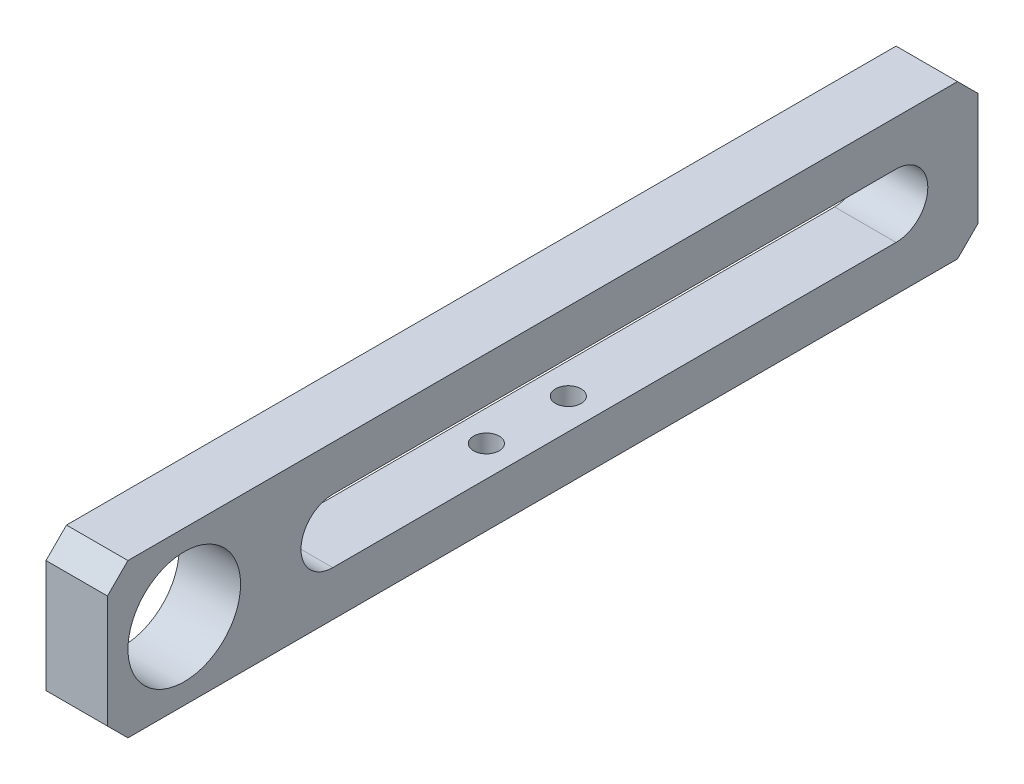
from build123d import *

# Parameters (mm, degrees)
SKETCH1_W              = 85
SKETCH1_H              = 15
EXTRUDE1_DEPTH         = 6
M12X1_0_TAPPED_HOLE1_D = 11
CHAMFER1_SIZE          = 2
M3_TAPPED_HOLE1_D      = 2.5
M3_TAPPED_HOLE1_DEPTH  = 8.5
M3_TAPPED_HOLE1_TIP    = 0.751075774


with BuildPart() as part:
    # Sketch1 → Extrude1 (new body)
    with BuildSketch(Plane(origin=(0, 0, 0), x_dir=(0, 0, -1), z_dir=(1, 0, 0))):
        with Locations((42.5, -7.5)):
            Rectangle(SKETCH1_W, SKETCH1_H)
        with BuildLine():
            Line((22, -4.4), (77, -4.4))
            ThreePointArc((77, -4.4), (80.1, -7.5), (77, -10.6))
            Line((77, -10.6), (22, -10.6))
            ThreePointArc((22, -10.6), (18.9, -7.5), (22, -4.4))
        make_face(mode=Mode.SUBTRACT)
    extrude(amount=EXTRUDE1_DEPTH)

    # M12x1.0 Tapped Hole1 (through all)
    with Locations(Plane(origin=(6, 0, 0), x_dir=(0, 0, -1), z_dir=(1, 0, 0))):
        with Locations((7.5, -7.5)):
            Hole(M12X1_0_TAPPED_HOLE1_D / 2)

    # Chamfer1
    chamfer1_edges = [part.edges().sort_by_distance(p)[0] for p in [
        (3, 0, 0),
        (3, 0, -85),
        (3, -15, -85),
        (3, -15, 0),
    ]]
    chamfer(chamfer1_edges, length=CHAMFER1_SIZE)

    # M3 Tapped Hole1
    with Locations(Plane.XZ.offset(15)):
        with Locations((3, -40), (3, -48)):
            Hole(M3_TAPPED_HOLE1_D / 2, depth=M3_TAPPED_HOLE1_DEPTH)
            with Locations((0, 0, -(M3_TAPPED_HOLE1_DEPTH + M3_TAPPED_HOLE1_TIP / 2))):  # 118° drill point
                Cone(0, M3_TAPPED_HOLE1_D / 2, M3_TAPPED_HOLE1_TIP, mode=Mode.SUBTRACT)


solid = part.part
